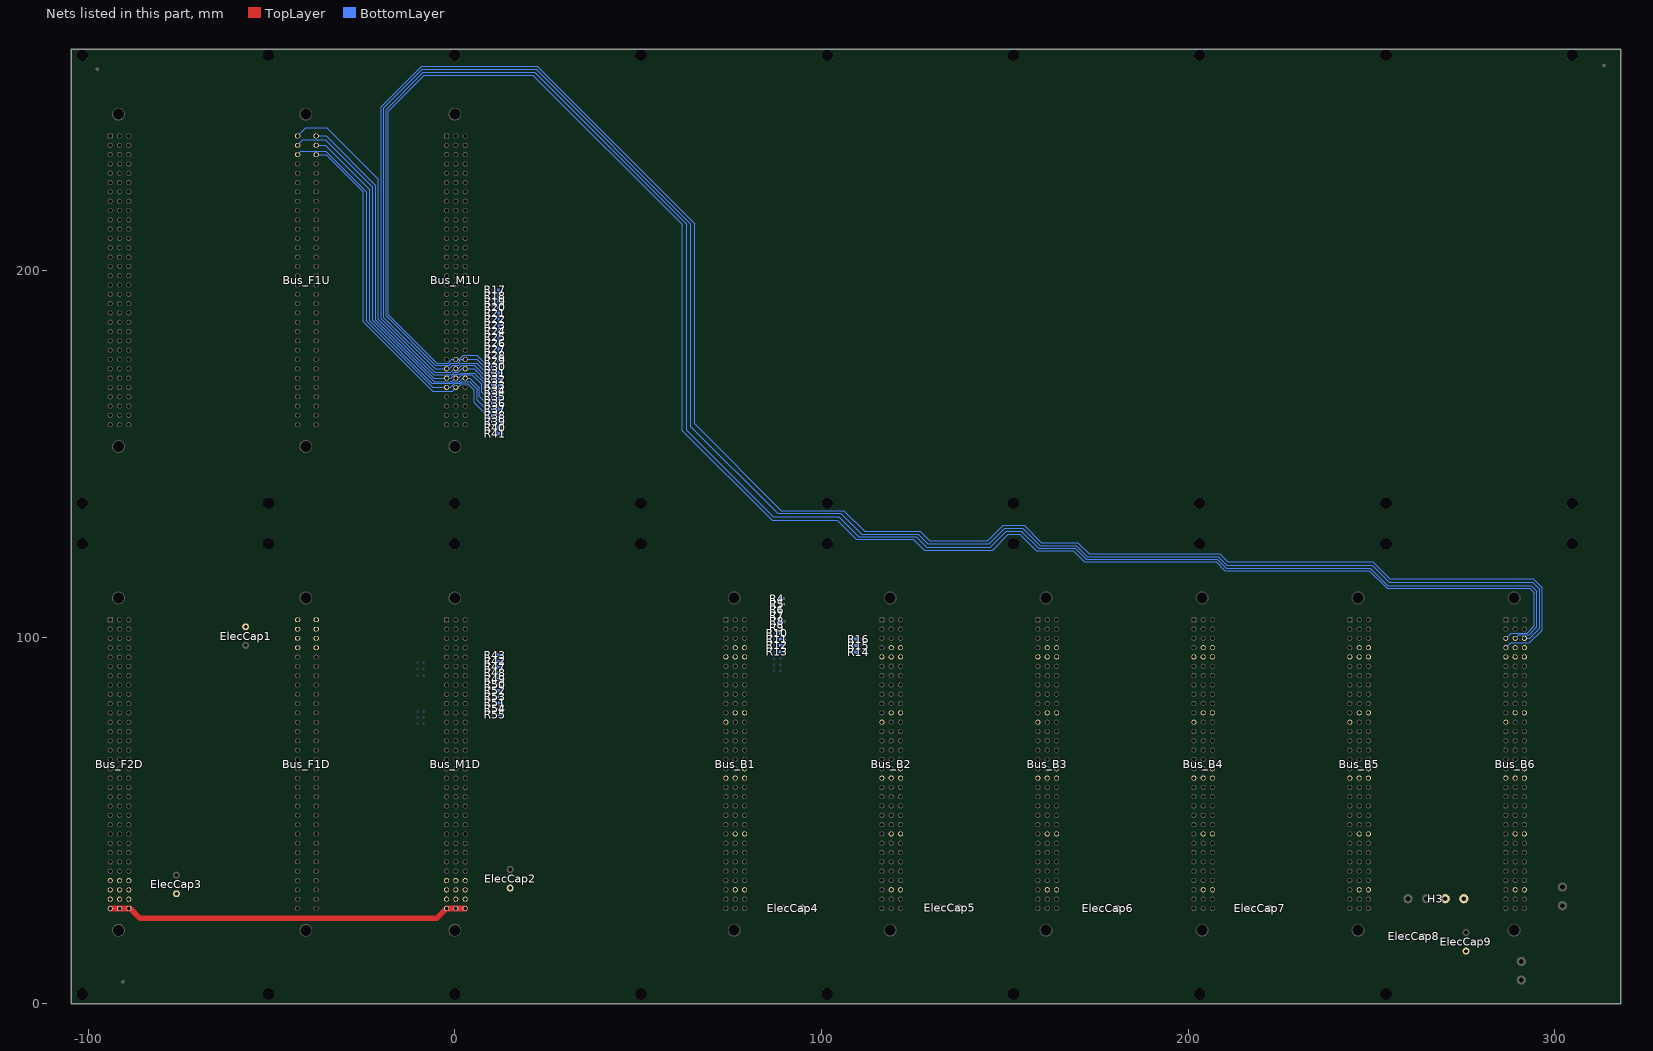
[diagram p0: the nets of this part, all layers, seen from the top]
# Altium PCB MISC67337.PcbDoc (part 7 of 7)
Units mm, origin at the board's own origin, x right, y up, seen from the top; angles counter-clockwise.
Board outline 422.71 x 260.35 mm, 4 copper layers (TopLayer, InternalPlane1, InternalPlane2, BottomLayer); 82 components, 143 nets, 1295 pads, 42 vias.

## Via types
v1: diameter 0.61, hole 0.305, TopLayer to BottomLayer, 42 vias

## Nets (pads, with @x,y where several pads share a name; then routed paths per layer and width w, separated by ;. In a path a pad name is that pad's centre, name@x,y a point inside that pad or via, vN(x,y) a via of type N, cw(c..) or ccw(c..) an arc to the next point about the centre after c; other vN are vias at no path point) (continued)
BZT21: Bus_B6.A3 Bus_M1U.B25 R30.1 | length 521.3
  BottomLayer w0.254: R30.1@10.262,173.685 9.195,173.685 6.031,176.849 2.351,176.849 1.195,175.693 Bus_M1U.B25@0.3,175.693 -0.857,175.693 -1.835,174.716 -4.866,174.716 -18.085,187.935 -18.085,243.459 -8.28,253.263 21.336,253.263 62.078,212.522 62.078,156.312 86.563,131.826 104.267,131.826 109.474,126.619 125.12,126.619 128.041,123.698 146.71,123.698 151.028,128.016 154.051,128.016 158.572,123.495 168.681,123.495 171.653,120.523 207.645,120.523 210.083,118.085 249.479,118.085 254.279,113.284 293.205,113.284 294.475,112.014 294.475,103.086 292.481,101.092 288.144,101.092 Bus_B6.A3@286.685,99.633
BZT22: Bus_B6.B3 Bus_M1U.C25 R31.2 | length 523.2
  BottomLayer w0.254: R31.2@10.262,171.983 9.754,171.983 6.044,175.693 Bus_M1U.C25@2.84,175.693 1.83,175.693 0.853,174.716 -0.925,174.716 -1.51,174.131 -5.272,174.131 -18.72,187.579 -18.72,243.865 -8.56,254.025 21.844,254.025 63.322,212.547 63.322,156.439 86.919,132.842 104.775,132.842 110.236,127.381 125.882,127.381 128.778,124.485 145.999,124.485 150.419,128.905 154.559,128.905 159.309,124.155 169.291,124.155 172.237,121.209 208.026,121.209 210.439,118.796 249.682,118.796 254.432,114.046 293.624,114.046 295.148,112.522 295.148,102.743 293.016,100.611 290.203,100.611 Bus_B6.B3@289.225,99.633
BZT23: Bus_B6.C3 Bus_M1U.A26 R32.2 | length 525.1
  BottomLayer w0.254: R32.2@10.262,170.332 5.969,174.625 1.524,174.625 1.03,174.131 -0.494,174.131 -1.472,173.153 Bus_M1U.A26@-2.24,173.153 -5.361,173.153 -19.329,187.122 -19.329,244.323 -8.839,254.813 22.2,254.813 64.389,212.623 64.389,157.404 88.062,133.731 105.283,133.731 110.998,128.016 126.441,128.016 129.057,125.4 145.771,125.4 150.038,129.667 154.94,129.667 159.664,124.943 169.57,124.943 172.568,121.945 208.229,121.945 210.591,119.583 250.215,119.583 254.864,114.935 294.005,114.935 295.961,112.979 295.961,102.413 293.181,99.633 Bus_B6.C3@291.765,99.633
BZT24: Bus_B6.A4 Bus_M1U.B26 R33.1 | length 536.5
  BottomLayer w0.254: R33.1@10.262,168.732 9.144,169.85 9.144,170.307 5.32,174.131 1.919,174.131 0.941,173.153 Bus_M1U.B26@0.3,173.153 -0.075,173.153 -1.052,172.176 -5.399,172.176 -20.015,186.792 -20.015,244.653 -9.017,255.651 22.504,255.651 65.405,212.75 65.405,158.115 89.027,134.493 106.045,134.493 111.76,128.778 126.975,128.778 129.515,126.238 145.364,126.238 149.555,130.429 155.321,130.429 160.02,125.73 169.926,125.73 172.999,122.657 208.712,122.657 210.845,120.523 250.419,120.523 254.991,115.951 294.132,115.951 296.596,113.487 296.596,101.905 293.116,98.425 288.017,98.425 Bus_B6.A4@286.685,97.093
GND: Bus_B1.A5 Bus_B1.A12 Bus_B1.A18 Bus_B1.B4 Bus_B1.B5 Bus_B1.B11 Bus_B1.B18 Bus_B1.B24 Bus_B1.B30 Bus_B1.C4 Bus_B1.C5 Bus_B1.C11 Bus_B1.C17 Bus_B1.C18 Bus_B1.C24 Bus_B1.C30 Bus_B2.A5 Bus_B2.A12 Bus_B2.A18 Bus_B2.B4 Bus_B2.B5 Bus_B2.B11 Bus_B2.B18 Bus_B2.B24 Bus_B2.B30 Bus_B2.C4 Bus_B2.C5 Bus_B2.C11 Bus_B2.C17 Bus_B2.C18 Bus_B2.C24 Bus_B2.C30 Bus_B3.A5 Bus_B3.A12 Bus_B3.A18 Bus_B3.B4 Bus_B3.B5 Bus_B3.B11 Bus_B3.B18 Bus_B3.B24 Bus_B3.B30 Bus_B3.C4 Bus_B3.C5 Bus_B3.C11 Bus_B3.C17 Bus_B3.C18 Bus_B3.C24 Bus_B3.C30 Bus_B4.A5 Bus_B4.A12 Bus_B4.A18 Bus_B4.B4 Bus_B4.B5 Bus_B4.B11 Bus_B4.B18 Bus_B4.B24 Bus_B4.B30 Bus_B4.C4 Bus_B4.C5 Bus_B4.C11 Bus_B4.C17 Bus_B4.C18 Bus_B4.C24 Bus_B4.C30 Bus_B5.A5 Bus_B5.A12 Bus_B5.A18 Bus_B5.B4 Bus_B5.B5 Bus_B5.B11 Bus_B5.B18 Bus_B5.B24 Bus_B5.B30 Bus_B5.C4 Bus_B5.C5 Bus_B5.C11 Bus_B5.C17 Bus_B5.C18 Bus_B5.C24 Bus_B5.C30 Bus_B6.A5 Bus_B6.A12 Bus_B6.A18 Bus_B6.B4 Bus_B6.B5 Bus_B6.B11 Bus_B6.B18 Bus_B6.B24 Bus_B6.B30 Bus_B6.C4 Bus_B6.C5 Bus_B6.C11 Bus_B6.C17 Bus_B6.C18 Bus_B6.C24 Bus_B6.C30 Bus_F1D.A1 Bus_F1D.A2 Bus_F1D.A3 Bus_F1D.A4 Bus_F1D.C1 Bus_F1D.C2 Bus_F1D.C3 Bus_F1D.C4 Bus_F2D.A29 Bus_F2D.A30 Bus_F2D.A31 Bus_F2D.B29 Bus_F2D.B30 Bus_F2D.B31 Bus_F2D.C29 Bus_F2D.C30 Bus_F2D.C31 Bus_M1D.A29 Bus_M1D.A30 Bus_M1D.A31 Bus_M1D.B29 Bus_M1D.B30 Bus_M1D.B31 Bus_M1D.C29 Bus_M1D.C30 Bus_M1D.C31 ElecCap1.2 ElecCap2.2 ElecCap3.2 ElecCap4.2 ElecCap5.2 ElecCap6.2 ElecCap7.2 ElecCap8.2 ElecCap9.2 H3.3 H3.4 R4.1 R5.2 R6.1 R7.1 R8.2 R9.1 R10.1 R11.1 R12.2 R13.1 R14.1 R15.2 R16.1 R17.1 R18.2 R19.1 R20.1 R21.2 R22.1 R23.1 R24.2 R25.1 R26.1 R27.2 R28.1 R29.1 R30.2 R31.1 R32.1 R33.2 R34.1 R35.1 R36.2 R37.1 R38.1 R39.2 R40.1 R41.1 R42.2 R43.1 R47.1 R48.2 R49.1 R50.1 R51.1 R52.2 R53.1 R54.1 R55.2 | length 85.7
  TopLayer w0.254: Bus_B1.C30@79.04,31.053 Bus_B1.C30@79.356,31.369 ; Bus_B3.C30@164.13,30.926 Bus_B3.C30@164.446,31.242
  BottomLayer w0.508: R55.2@11.862,78.765 v1(12.802,78.765) ; R54.1@11.862,80.391 v1(12.827,80.391) ; R51.1@11.862,82.042 12.827,82.042 v1(12.852,82.017) ; R53.1@11.862,83.693 v1(12.852,83.693) ; R52.2@11.862,85.395 v1(12.878,85.395) ; R50.1@11.862,86.995 v1(12.827,86.995) ; R49.1@11.862,88.494 v1(12.827,88.494) ; R48.2@11.862,90.195 v1(12.878,90.195) ; R47.1@11.862,91.821 12.878,91.821 v1(12.903,91.796) ; R42.2@11.862,93.37 v1(12.852,93.37) ; R43.1@11.862,95.047 v1(12.903,95.047) ; R17.1@11.938,194.666 R18.2@11.938,193.065 R19.1@11.938,191.491 R20.1@11.938,189.916 R21.2@11.938,188.316 R22.1@11.938,186.69 R23.1@11.938,185.064 R24.2@11.938,183.388 ; v1(12.852,167.107) R34.1@11.938,167.107 ; v1(12.852,170.332) R32.1@11.938,170.332 ; v1(12.878,165.481) R35.1@11.938,165.481 ; v1(12.878,168.758) 12.852,168.732 R33.2@11.938,168.732 ; v1(12.878,171.983) R31.1@11.938,171.983 ; v1(12.878,173.685) R30.2@11.938,173.685 ; v1(12.903,160.452) R38.1@11.938,160.452 ; v1(12.903,163.805) R36.2@11.938,163.805 ; v1(12.903,175.311) R29.1@11.938,175.311 ; v1(12.903,176.886) R28.1@11.938,176.886 ; v1(12.903,178.537) R27.2@11.938,178.537 ; v1(12.903,180.162) R26.1@11.938,180.162 ; v1(12.903,181.762) R25.1@11.938,181.762 ; v1(12.929,155.473) R41.1@11.938,155.473 R40.1@11.938,157.124 ; v1(12.929,162.154) R37.1@11.938,162.154 ; v1(12.954,157.124) R40.1@11.938,157.124 ; v1(12.954,158.775) R39.2@11.938,158.775 ; v1(12.954,183.388) R24.2@11.938,183.388 ; R13.1@88.773,95.936 89.865,95.936 89.916,95.885 v1(89.916,95.936) ; R12.2@88.773,97.79 v1(89.916,97.79) ; R10.1@88.773,100.965 R11.1@88.773,99.39 v1(89.891,99.39) ; R9.1@88.773,102.565 R8.2@88.773,104.242 v1(89.865,104.242) ; R7.1@88.773,105.842 R6.1@88.773,107.442 R5.2@88.773,108.991 89.764,108.991 v1(89.789,108.966) ; R4.1@88.773,110.49 v1(89.789,110.49) ; v1(107.95,95.885) R14.1@109.372,95.885 ; v1(107.95,97.663) R15.2@109.372,97.663 ; v1(107.95,99.441) R16.1@109.372,99.441 ; R40.1@11.938,157.124 R39.2@11.938,158.775 ; R39.2@11.938,158.775 R38.1@11.938,160.452 ; R38.1@11.938,160.452 R37.1@11.938,162.154 ; R37.1@11.938,162.154 R36.2@11.938,163.805 ; R36.2@11.938,163.805 R35.1@11.938,165.481 ; R35.1@11.938,165.481 R34.1@11.938,167.107 ; R34.1@11.938,167.107 R33.2@11.938,168.732 ; R33.2@11.938,168.732 R32.1@11.938,170.332 ; R32.1@11.938,170.332 R31.1@11.938,171.983 ; R31.1@11.938,171.983 R30.2@11.938,173.685 ; R30.2@11.938,173.685 R29.1@11.938,175.311 ; R29.1@11.938,175.311 R28.1@11.938,176.886 ; R28.1@11.938,176.886 R27.2@11.938,178.537 ; R27.2@11.938,178.537 R26.1@11.938,180.162 ; R26.1@11.938,180.162 R25.1@11.938,181.762 ; R25.1@11.938,181.762 R24.2@11.938,183.388
IPR1: Bus_F1U.C2 Bus_M1U.C27 R37.2 | length 101.3
  BottomLayer w0.254: Bus_F1U.C2@-37.8,234.113 -35.358,234.113 -23.241,221.996 -23.241,186.258 -6.212,169.229 -0.635,169.229 -0.229,169.636 1.234,169.636 2.211,170.613 Bus_M1U.C27@2.84,170.613 4.139,170.613 6.731,168.021 6.731,165.684 R37.2@10.262,162.154
IPR2: Bus_F1U.A3 Bus_M1U.A28 R38.2 | length 107.1
  BottomLayer w0.254: Bus_F1U.A3@-42.88,231.573 -41.966,232.488 -35.13,232.488 -24.003,221.361 -24.003,186.131 -5.945,168.073 Bus_M1U.A28@-2.24,168.073 -1.091,168.073 0,169.164 1.456,169.164 1.927,169.636 4.1,169.636 6.096,167.64 6.096,164.617 R38.2@10.262,160.452
IPR3: Bus_F1U.C3 Bus_M1U.B28 R39.1 | length 102.7
  BottomLayer w0.254: Bus_F1U.C3@-37.8,231.573 -35.104,231.573 -24.943,221.412 -24.943,186.004 -6.034,167.096 -0.678,167.096 Bus_M1U.B28@0.3,168.073 0.94,168.073 1.918,169.051 3.542,169.051 5.334,167.259 5.334,163.83 10.262,158.902 R39.1@10.262,158.775
PG: Bus_F2D.A32 Bus_F2D.B32 Bus_F2D.C32 Bus_M1D.A32 Bus_M1D.B32 Bus_M1D.C32 | length 99.1
  TopLayer w1.524: Bus_F2D.A32@-93.97,25.954 Bus_F2D.B32@-91.43,25.954 Bus_F2D.C32@-88.89,25.954 -88.519,25.954 -85.806,23.241 -4.953,23.241 Bus_M1D.A32@-2.24,25.954 Bus_M1D.B32@0.3,25.954 Bus_M1D.C32@2.84,25.954
UPR1: Bus_F1U.A1 Bus_M1U.C26 R34.2 | length 108.1
  BottomLayer w0.254: Bus_F1U.A1@-42.88,236.653 -40.646,238.887 -34.925,238.887 -20.853,224.815 -20.853,186.665 -5.78,171.591 -0.787,171.591 -0.203,172.176 0.98,172.176 1.957,173.153 Bus_M1U.C26@2.84,173.153 5.282,173.153 8.509,169.926 8.509,169.037 10.236,167.31 10.236,167.132 R34.2@10.262,167.107
UPR2: Bus_F1U.C1 Bus_M1U.A27 R35.2 | length 101.3
  BottomLayer w0.254: Bus_F1U.C1@-37.8,236.653 -35.104,236.653 -21.59,223.139 -21.59,186.461 -5.742,170.613 Bus_M1U.A27@-2.24,170.613 -1.091,170.613 0,171.704 1.456,171.704 1.749,171.998 5.294,171.998 8.001,169.291 8.001,167.742 R35.2@10.262,165.481 R35.2@10.135,165.608
UPR3: Bus_F1U.A2 Bus_M1U.B27 R36.1 | length 107.7
  BottomLayer w0.254: Bus_F1U.A2@-42.88,234.113 -41.408,235.585 -35.306,235.585 -22.352,222.631 -22.352,186.334 -5.653,169.636 -0.803,169.636 0.175,170.613 Bus_M1U.B27@0.3,170.613 0.94,170.613 1.918,171.591 4.685,171.591 7.366,168.91 7.366,166.7 R36.1@10.262,163.805
pads on no net: Bus_B1.0 Bus_B2.0 Bus_B3.0 Bus_B4.0 Bus_B5.0 Bus_B6.0 Bus_F1D.0 Bus_F1D.A9 Bus_F1D.A10 Bus_F1D.A11 Bus_F1D.A12 Bus_F1D.A13 Bus_F1D.A14 Bus_F1D.A15 Bus_F1D.A16 Bus_F1D.A17 Bus_F1D.A18 Bus_F1D.A19 Bus_F1D.A20 Bus_F1D.A21 Bus_F1D.A22 Bus_F1D.A23 Bus_F1D.A24 Bus_F1D.A25 Bus_F1D.A26 Bus_F1D.A27 Bus_F1D.A28 Bus_F1D.A29 Bus_F1D.A30 Bus_F1D.A31 Bus_F1D.A32 Bus_F1D.C9 Bus_F1D.C10 Bus_F1D.C11 Bus_F1D.C12 Bus_F1D.C13 Bus_F1D.C14 Bus_F1D.C15 Bus_F1D.C16 Bus_F1D.C17 Bus_F1D.C18 Bus_F1D.C19 Bus_F1D.C20 Bus_F1D.C21 Bus_F1D.C22 Bus_F1D.C23 Bus_F1D.C24 Bus_F1D.C25 Bus_F1D.C26 Bus_F1D.C27 Bus_F1D.C28 Bus_F1D.C29 Bus_F1D.C30 Bus_F1D.C31 Bus_F1D.C32 Bus_F1U.0 Bus_F1U.A4 Bus_F1U.A5 Bus_F1U.A6 Bus_F1U.A7 Bus_F1U.A8 Bus_F1U.A9 Bus_F1U.A10 Bus_F1U.A11 Bus_F1U.A12 Bus_F1U.A13 Bus_F1U.A14 Bus_F1U.A15 Bus_F1U.A16 Bus_F1U.A17 Bus_F1U.A18 Bus_F1U.A19 Bus_F1U.A20 Bus_F1U.A21 Bus_F1U.C4 Bus_F1U.C5 Bus_F1U.C6 Bus_F1U.C7 Bus_F1U.C8 Bus_F1U.C9 Bus_F1U.C10 Bus_F1U.C11 Bus_F1U.C12 Bus_F1U.C13 Bus_F1U.C14 Bus_F1U.C15 Bus_F1U.C16 Bus_F1U.C17 Bus_F1U.C18 Bus_F1U.C19 Bus_F1U.C20 Bus_F2D.0 Bus_F2D.A1 Bus_F2D.A2 Bus_F2D.A3 Bus_F2D.A4 Bus_F2D.A5 Bus_F2D.A6 Bus_F2D.A9 Bus_F2D.A10 Bus_F2D.A25 Bus_F2D.B1 Bus_F2D.B2 Bus_F2D.B3 Bus_F2D.B4 Bus_F2D.B5 Bus_F2D.B6 Bus_F2D.B9 Bus_F2D.B10 Bus_F2D.B18 Bus_F2D.B24 Bus_F2D.B25 Bus_F2D.C1 Bus_F2D.C2 Bus_F2D.C3 Bus_F2D.C4 Bus_F2D.C5 Bus_F2D.C6 Bus_F2D.C9 Bus_F2D.C11 Bus_F2D.C18 Bus_F2D.C24 Bus_F2D.C25 Bus_F2U.0 Bus_F2U.A1 Bus_F2U.A15 Bus_F2U.A16 Bus_F2U.A17 Bus_F2U.A18 Bus_F2U.A19 Bus_F2U.A20 Bus_F2U.A21 Bus_F2U.A22 Bus_F2U.A23 Bus_F2U.A24 Bus_F2U.A25 Bus_F2U.A26 Bus_F2U.A27 Bus_F2U.A28 Bus_F2U.A29 Bus_F2U.A30 Bus_F2U.A31 Bus_F2U.A32 Bus_F2U.B1 Bus_F2U.B8 Bus_F2U.B14 Bus_F2U.B15 Bus_F2U.B16 Bus_F2U.B17 Bus_F2U.B18 Bus_F2U.B19 Bus_F2U.B20 Bus_F2U.B21 Bus_F2U.B22 Bus_F2U.B23 Bus_F2U.B24 Bus_F2U.B25 Bus_F2U.B26 Bus_F2U.B27 Bus_F2U.B28 Bus_F2U.B29 Bus_F2U.B30 Bus_F2U.B31 Bus_F2U.B32 Bus_F2U.C1 Bus_F2U.C8 Bus_F2U.C14 Bus_F2U.C15 Bus_F2U.C16 Bus_F2U.C17 Bus_F2U.C18 Bus_F2U.C19 Bus_F2U.C20 Bus_F2U.C21 Bus_F2U.C22 Bus_F2U.C23 Bus_F2U.C24 Bus_F2U.C25 Bus_F2U.C26 Bus_F2U.C27 Bus_F2U.C28 Bus_F2U.C29 Bus_F2U.C30 Bus_F2U.C31 Bus_F2U.C32 Bus_M1D.0 Bus_M1D.A9 Bus_M1D.A25 Bus_M1D.B9 Bus_M1D.B18 Bus_M1D.B24 Bus_M1D.B25 Bus_M1D.C11 Bus_M1D.C18 Bus_M1D.C24 Bus_M1D.C25 Bus_M1U.0 Bus_M1U.A1 Bus_M1U.A15 Bus_M1U.A18 Bus_M1U.A30 Bus_M1U.A31 Bus_M1U.A32 Bus_M1U.B1 Bus_M1U.B8 Bus_M1U.B14 Bus_M1U.B15 Bus_M1U.B18 Bus_M1U.B29 Bus_M1U.B30 Bus_M1U.B31 Bus_M1U.B32 Bus_M1U.C1 Bus_M1U.C8 Bus_M1U.C14 Bus_M1U.C15 Bus_M1U.C29 Bus_M1U.C30 Bus_M1U.C31 Bus_M1U.C32

## Polygon pours and split planes (outlines as drawn)
+5V on BottomLayer "TopLayer-No Net" (solid, remove dead copper, pour order 1008): 272.542,20.93 272.542,19.025 272.542,18.644 272.745,18.44 273.101,18.085 274.168,18.085 280.365,18.085 282.55,20.269 286.817,24.536 289.585,24.536 292.43,24.536 293.116,25.222 293.649,25.756 293.649,26.797 293.649,28.677 293.091,29.235 292.786,29.54 292.608,29.718 286.055,29.718 284.277,29.718 282.905,28.346 277.825,23.266 275.869,23.266 273.761,23.266 273.761,23.063 272.618,21.92 272.542,21.844 272.542,20.93
+5V on BottomLayer "TopLayer-No Net" (solid, remove dead copper, pour order 1007): 242.519,28.626 242.519,24.435 242.824,24.13 243.789,23.165 246.431,23.165 248.818,23.165 255.702,16.281 256.642,15.342 259.182,15.342 259.359,15.342 260.045,16.027 260.375,16.358 260.375,17.78 260.375,21.234 254,27.61 252.07,29.54 248.412,29.54 243.434,29.54 242.519,28.626
+5V on BottomLayer "TopLayer-No Net" (solid, remove dead copper, pour order 1006): 200,28.194 200,24.613 200.304,24.308 200.99,23.622 202.692,23.622 217.78,23.622 217.932,23.774 218.389,24.232 218.389,25.425 218.389,27.457 217.856,27.991 216.205,29.642 216.154,29.693 216.129,29.718 201.676,29.718 200.812,29.718 200.381,29.286 200,28.905 200,28.194
+5V on BottomLayer "TopLayer-No Net" (solid, remove dead copper, pour order 1005): 157.556,27.915 157.556,25.146 157.81,24.892 159.08,23.622 167.818,23.622 176.2,23.622 176.733,24.155 177.19,24.613 177.19,26.086 177.19,26.949 176.352,27.788 174.498,29.642 162.382,29.642 158.217,29.642 157.683,29.108 157.556,28.981 157.556,27.915
+5V on BottomLayer "TopLayer-No Net" (solid, remove dead copper, pour order 1004): 114.833,27.889 114.808,27.864 114.808,24.79 114.808,24.536 115.24,24.105 116.027,23.317 126.009,23.317 133.426,23.317 133.807,23.698 134.137,24.028 134.137,25.781 134.137,26.746 133.121,27.762 131.394,29.489 121.361,29.489 115.595,29.489 115.011,28.905 114.833,28.727 114.833,27.889
+5V on BottomLayer "TopLayer-No Net" (solid, remove dead copper, pour order 1003): 72.415,28.219 72.415,24.282 73,23.698 90.322,23.698 91.084,24.46 91.237,24.613 91.237,26.264 91.237,27.381 91.237,27.965 89.738,29.464 72.847,29.464 72.466,29.083 72.415,29.032 72.415,28.219
+5V on BottomLayer "TopLayer-No Net" (solid, remove dead copper, pour order 1002): -3.658,41.3 -3.658,40.945 -3.658,35.966 -3.15,35.458 -2.743,35.052 0.051,35.052 16.18,35.052 16.713,35.585 16.713,36.855 16.713,39.319 15.773,40.259 13.818,42.215 -2.337,42.215 -3.15,42.215 -3.175,42.215 -3.632,41.758 -3.658,41.732 -3.658,41.3
+5V on BottomLayer "TopLayer-No Net" (solid, remove dead copper, pour order 1001): -58.903,97.638 -58.903,91.364 -57.023,89.484 -53.543,86.004 -38.227,86.004 -37.008,86.004 -36.678,86.335 -36.195,86.817 -36.195,87.96 -36.195,94.463 -36.932,95.199 -37.236,95.504 -37.973,95.504 -47.549,95.504 -49.53,97.485 -51.359,99.314 -54.712,99.314 -58.344,99.314 -58.699,98.958 -58.903,98.755 -58.903,97.638
+5V on BottomLayer "TopLayer-No Net" (solid, remove dead copper, pour order 1000): -94.92,41.427 -94.92,39.294 -94.92,35.687 -94.539,35.306 -94.412,35.179 -93.802,35.179 -83.134,35.179 -82.804,34.849 -81.432,33.477 -78.715,33.477 -74.752,33.477 -74.32,33.909 -73.965,34.265 -73.965,35.687 -73.965,39.853 -73.965,40.132 -75.895,42.062 -94.59,42.062 -94.894,41.758 -94.92,41.732 -94.92,41.427
GND on InternalPlane1 (split plane): 317.555,0.51 -104.131,0.51 -104.131,259.84 317.555,259.84
+5V on InternalPlane2 (split plane): 317.555,0.51 -104.131,0.51 -104.131,259.84 317.555,259.84

## Keep-outs
KeepOutLayer:
  circle w0.254: c161.29,250.952 r1.5
  circle w0.254: c203.835,250.952 r1.5
  circle w0.254: c246.38,250.952 r1.5
  circle w0.254: c118.745,250.952 r1.5
  circle w0.254: c306.15,8.89 r6
  lines w0.254: -104.641,0 318.066,0 318.066,260.35 -104.641,260.35 -104.641,0

## Silkscreen, mask and mechanical layers (free items; w line width, h text height)
Mechanical1:
  circle w0.254: c246.38,9.398 r1.5
  circle w0.254: c203.835,9.398 r1.5
  circle w0.254: c161.29,9.398 r1.5
  circle w0.254: c118.745,9.398 r1.5